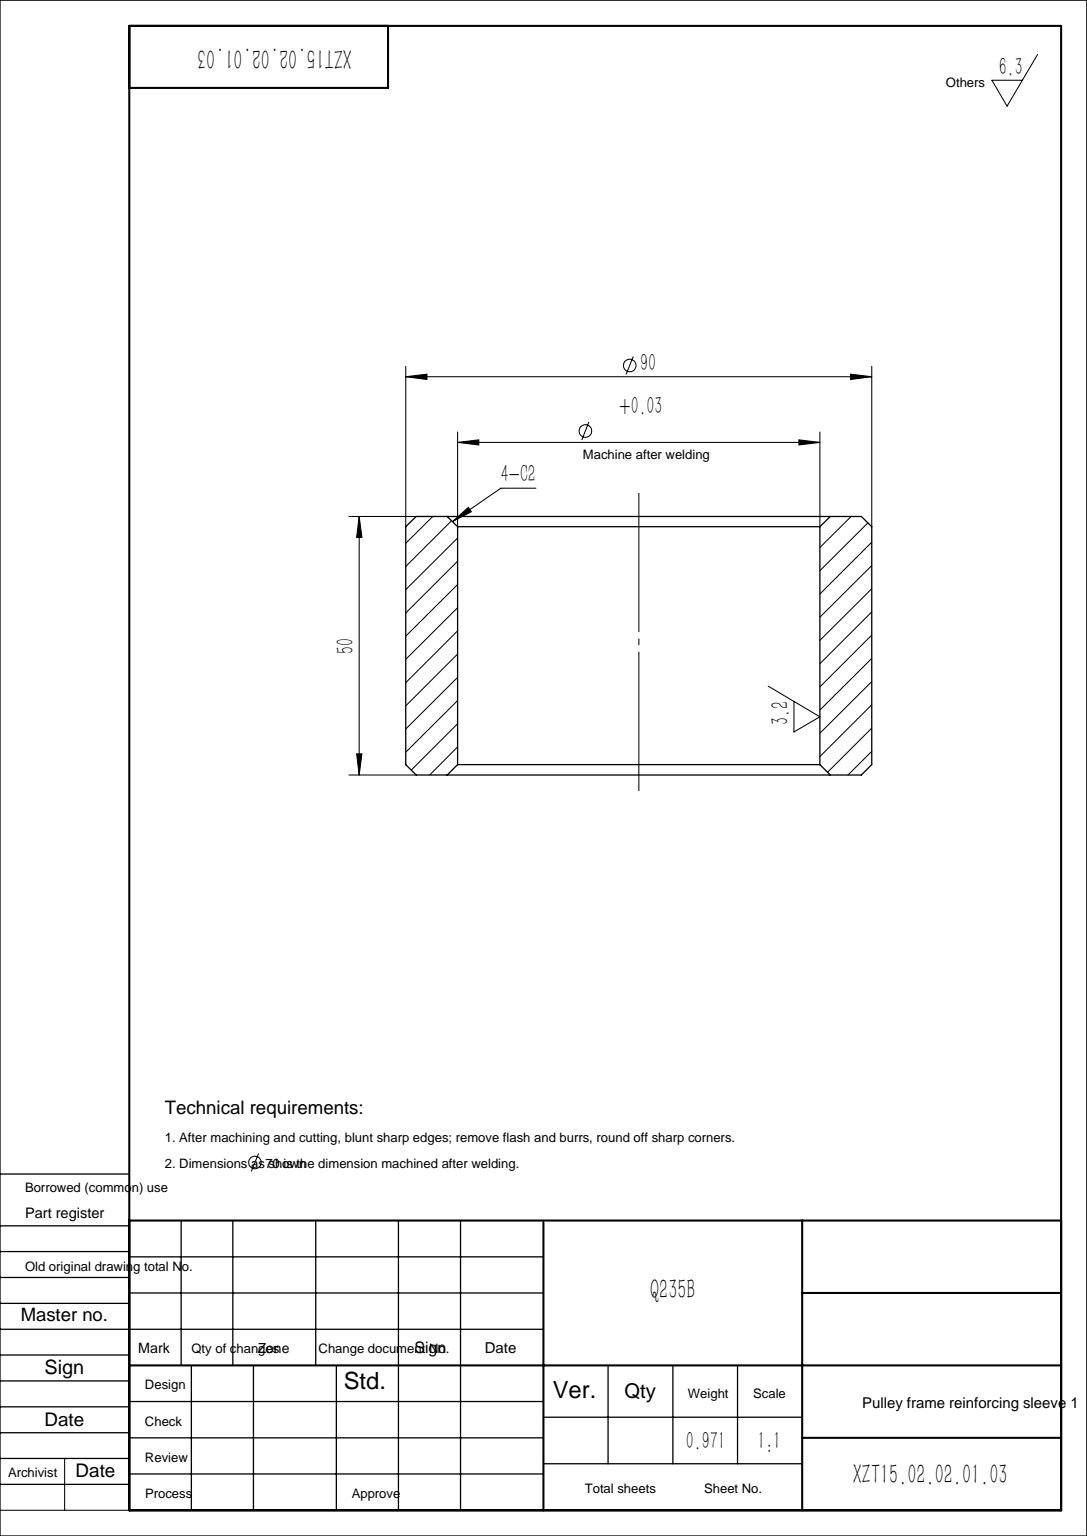
SolidWorks part; units mm, degrees
material "Q235B"
ref_plane "Front Plane" through (0, 0, 0) normal (0, 0, 1) x (1, 0, 0)
ref_plane "Top Plane" through (0, 0, 0) normal (0, 1, 0) x (1, 0, 0)
ref_plane "Right Plane" through (0, 0, 0) normal (1, 0, 0) x (0, 0, -1)
sketch "Sketch1" plane through (0, 0, 0) normal (0, 1, 0) x (1, 0, 0)
  circle A0 centre (0, 0) radius 35
  circle A1 centre (0, 0) radius 45
  dimension "D1" = 70
  dimension "D2" = 90
extrude "Boss-Extrude1" add sketch "Sketch1" along normal blind 50
chamfer "Chamfer2" distance 2 angle 45 4 edges at (0, 0, 35) (0, 50, 35) (0, 0, 45) (0, 50, 45)
